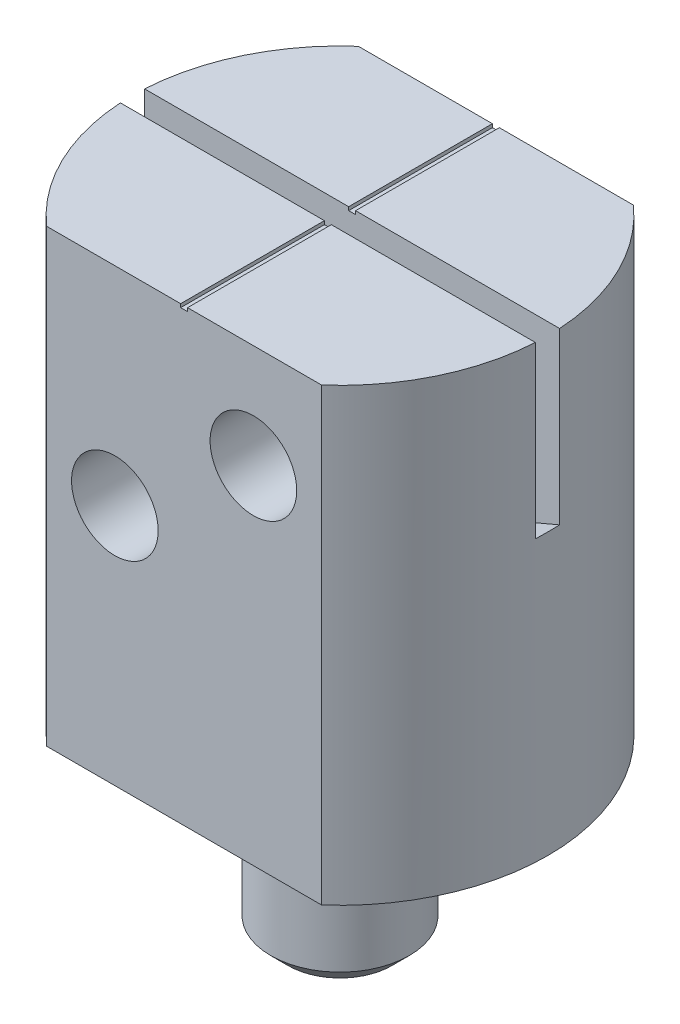
from build123d import *

# Parameters (mm, degrees)
SKETCH1_R           = 6
BOSS_EXTRUDE1_DEPTH = 18
SKETCH2_OUTSIDE_W   = 18.948
SKETCH2_OUTSIDE_H   = 18.948
SKETCH2_OUTSIDE_R   = 2
CUT_EXTRUDE1_DEPTH  = 5
CUT_EXTRUDE2_DEPTH  = 0.35
CHAMFER1_SIZE       = 0.5
SKETCH6_W           = 0.3
SKETCH6_H           = 0.3
SKETCH9_OUTSIDE_W   = 18.948
SKETCH9_OUTSIDE_H   = 18.948
SKETCH9_OUTSIDE_W_2 = 12.764596016
SKETCH9_OUTSIDE_H_2 = 9
CUT_EXTRUDE3_DEPTH  = 20.899748742
M3_TAPPED_HOLE1_D   = 2.5
SKETCH14_W          = 0.2
SKETCH14_H          = 9
CUT_EXTRUDE5_DEPTH  = 0.1


with BuildPart() as part:
    # Sketch1 → Boss-Extrude1 (new body)
    with BuildSketch(Plane(origin=(0, 0, 0), x_dir=(1, 0, 0), z_dir=(0, 1, 0))):
        with Locations(Location((0, 0, 0), (0, 0, 270))):
            Circle(SKETCH1_R)
    extrude(amount=BOSS_EXTRUDE1_DEPTH)

    # Sketch2 outside → Cut-Extrude1 (cut)
    with BuildSketch(Plane.XZ):
        Rectangle(SKETCH2_OUTSIDE_W, SKETCH2_OUTSIDE_H)
        with Locations(Location((0, 0, 0), (0, 0, 270))):
            Circle(SKETCH2_OUTSIDE_R, mode=Mode.SUBTRACT)
    extrude(amount=-CUT_EXTRUDE1_DEPTH, mode=Mode.SUBTRACT)

    # Sketch8 → Cut-Extrude2 (cut, symmetric)
    with BuildSketch(Plane.XY):
        Polygon((-6, 8), (6, 13.093697795), (6, 18), (-6, 18), align=None)
    extrude(amount=CUT_EXTRUDE2_DEPTH, both=True, mode=Mode.SUBTRACT)

    # Chamfer1
    chamfer1_edges = [part.edges().sort_by_distance(p)[0] for p in [
        (0, 0, 2),
    ]]
    chamfer(chamfer1_edges, length=CHAMFER1_SIZE)

    # Sketch6 → Cut-Revolve1 (revolve, cut)
    with BuildSketch(Plane.XY, mode=Mode.PRIVATE) as cut_revolve1_sk:
        with Locations((1.85, 4.85)):
            Rectangle(SKETCH6_W, SKETCH6_H)
    revolve(cut_revolve1_sk.sketch.rotate(Axis((0, 0, 0), (0, 1, 0)), 90), axis=Axis((0, 0, 0), (0, 1, 0)), mode=Mode.SUBTRACT)

    # Sketch9 outside → Cut-Extrude3 (cut, through all)
    with BuildSketch(Plane(origin=(0, 18, 0), x_dir=(1, 0, 0), z_dir=(0, 1, 0))):
        Rectangle(SKETCH9_OUTSIDE_W, SKETCH9_OUTSIDE_H)
        Rectangle(SKETCH9_OUTSIDE_W_2, SKETCH9_OUTSIDE_H_2, mode=Mode.SUBTRACT)
    extrude(amount=-CUT_EXTRUDE3_DEPTH, mode=Mode.SUBTRACT)

    # M3 Tapped Hole1 (through all)
    with Locations(Plane.XY.offset(4.5)):
        with Locations((2, 15), (-2, 12)):
            Hole(M3_TAPPED_HOLE1_D / 2)

    # Sketch14 → Cut-Extrude5 (cut)
    with BuildSketch(Plane(origin=(0, 18, 0), x_dir=(1, 0, 0), z_dir=(0, 1, 0))):
        Rectangle(SKETCH14_W, SKETCH14_H)
    extrude(amount=-CUT_EXTRUDE5_DEPTH, mode=Mode.SUBTRACT)


solid = part.part
